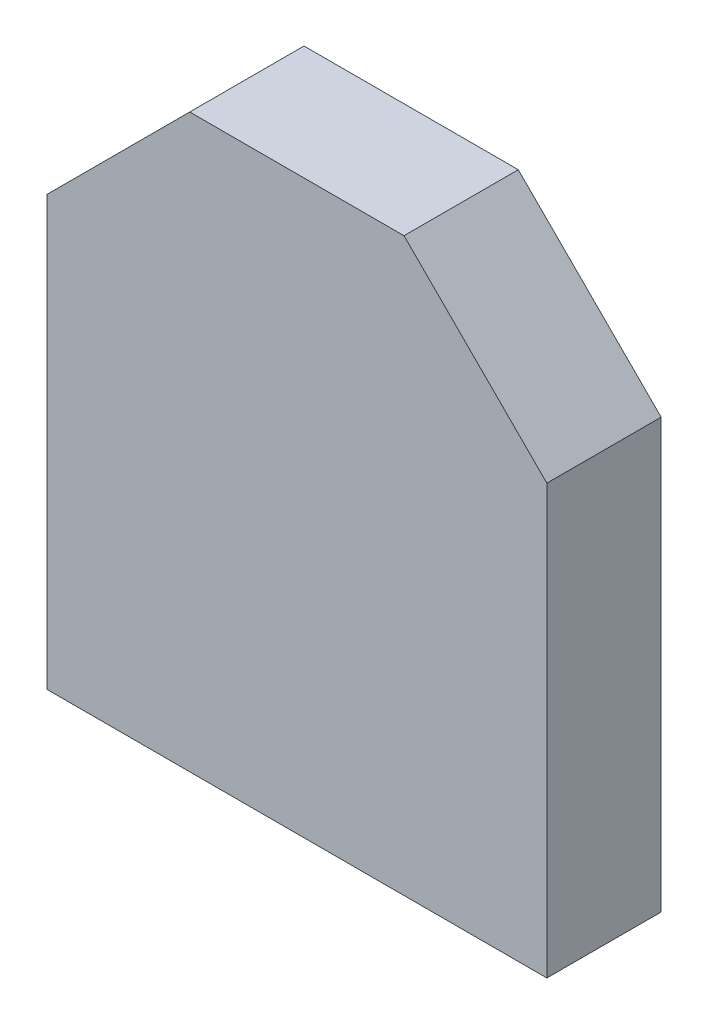
from build123d import *

# Parameters (mm, degrees)
BOSS_EXTRUDE1_DEPTH = 8


with BuildPart() as part:
    # Sketch1 → Boss-Extrude1 (new body)
    with BuildSketch(Plane.XY):
        Polygon((0, 30), (10, 40), (25, 40), (35, 30), (35, 0), (0, 0), align=None)
    extrude(amount=BOSS_EXTRUDE1_DEPTH)


solid = part.part
